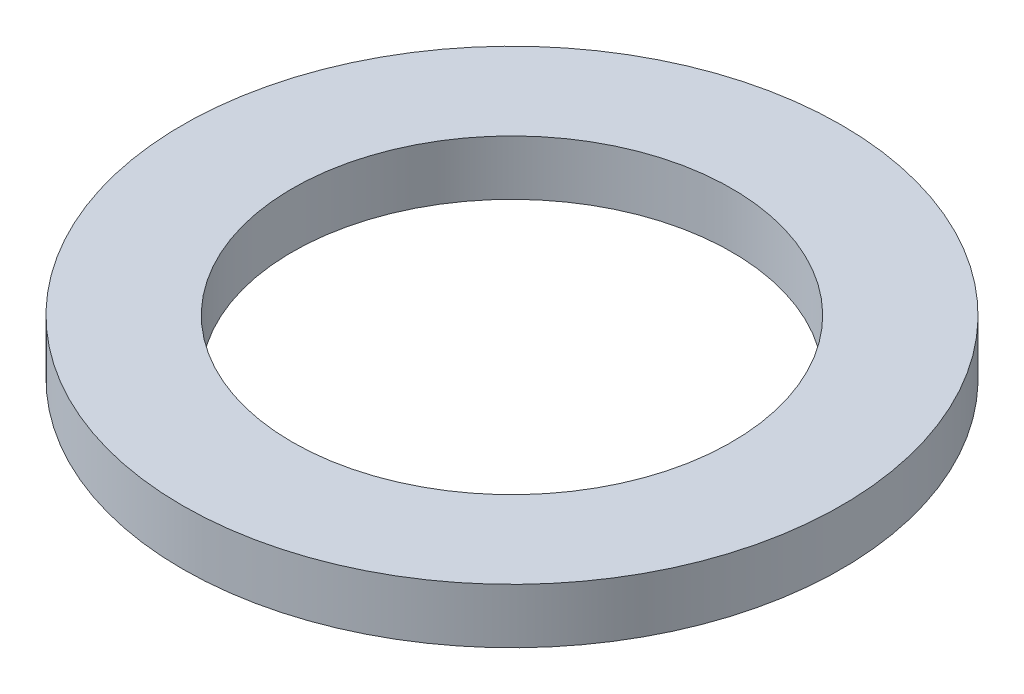
SolidWorks part; units mm, degrees
ref_plane "Front Plane" through (0, 0, 0) normal (0, 0, 1) x (1, 0, 0)
ref_plane "Top Plane" through (0, 0, 0) normal (0, 1, 0) x (1, 0, 0)
ref_plane "Right Plane" through (0, 0, 0) normal (1, 0, 0) x (0, 0, -1)
other "Configuration Table"
sketch "Sketch1" plane through (0, 0, 0) normal (0, 1, 0) x (1, 0, 0)
  circle A0 centre (0, 0) radius 12
  circle A1 centre (0, 0) radius 8
  dimension "D1" = 24
  dimension "D2" = 16
extrude "Boss-Extrude3" add sketch "Sketch1" along normal blind 2 contours A0 A1
